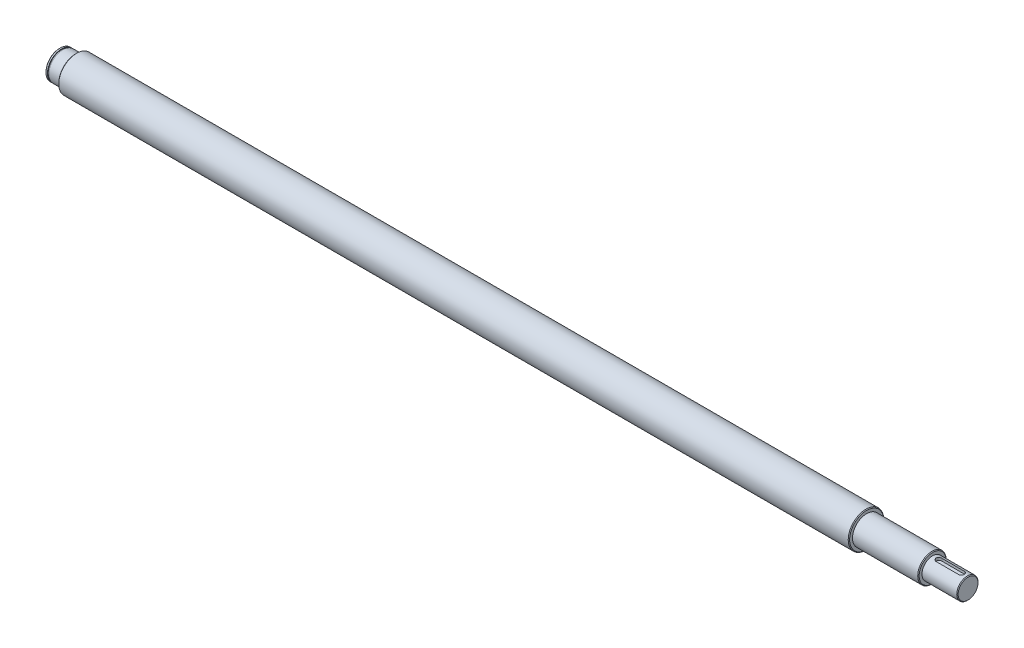
from build123d import *

# Parameters (mm, degrees)
CUT_EXTRUDE_1_DEPTH = 4


with BuildPart() as part:
    # 草图1 → 旋转1 (revolve)
    with BuildSketch(Plane.XY, mode=Mode.PRIVATE) as revolve_1_sk:
        with BuildLine():
            Line((0, 0), (0, 19))
            Line((0, 19), (1, 20))
            Line((1, 20), (3.05, 20))
            Line((3.05, 20), (3.05, 19))
            Line((3.05, 19), (5, 19))
            Line((5, 19), (5, 20))
            Line((5, 20), (22.75, 20))
            ThreePointArc((22.75, 20), (22.926776695, 20.073223305), (23, 20.25))
            Line((23, 20.25), (23, 24))
            Line((23, 24), (24, 25))
            Line((24, 25), (1137, 25))
            Line((1137, 25), (1138, 24))
            Line((1138, 24), (1138, 20))
            Line((1138, 20), (1230, 20))
            Line((1230, 20), (1231, 19))
            Line((1231, 19), (1231, 15))
            Line((1231, 15), (1280, 15))
            Line((1280, 15), (1281, 14))
            Line((1281, 14), (1281, 0))
            Line((1281, 0), (0, 0))
        make_face()
    revolve(revolve_1_sk.sketch.rotate(Axis((1281, 0, 0), (-1, 0, 0)), 270), axis=Axis((1281, 0, 0), (-1, 0, 0)))

    # 草图2 → 切除-拉伸1 (cut)
    with BuildSketch(Plane(origin=(0, 15, 0), x_dir=(1, 0, 0), z_dir=(0, 1, 0))):
        with BuildLine():
            Line((1240, -4), (1272, -4))
            ThreePointArc((1272, -4), (1276, 0), (1272, 4))
            Line((1272, 4), (1240, 4))
            ThreePointArc((1240, 4), (1236, 0), (1240, -4))
        make_face()
    extrude(amount=-CUT_EXTRUDE_1_DEPTH, mode=Mode.SUBTRACT)


solid = part.part
